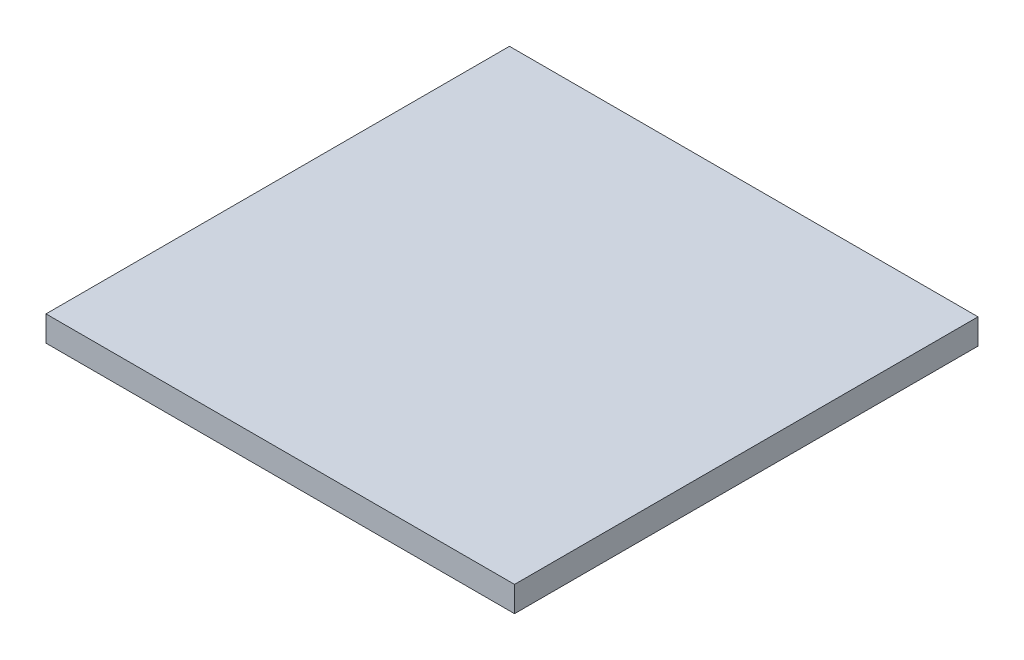
from build123d import *

# Parameters (mm, degrees)
SKETCH1_W           = 369
SKETCH1_H           = 365
BOSS_EXTRUDE1_DEPTH = 20


with BuildPart() as part:
    # Sketch1 → Boss-Extrude1 (new body)
    with BuildSketch(Plane(origin=(0, 0, 0), x_dir=(1, 0, 0), z_dir=(0, 1, 0))):
        with Locations((-184.5, 182.5)):
            Rectangle(SKETCH1_W, SKETCH1_H)
    extrude(amount=BOSS_EXTRUDE1_DEPTH)


solid = part.part
